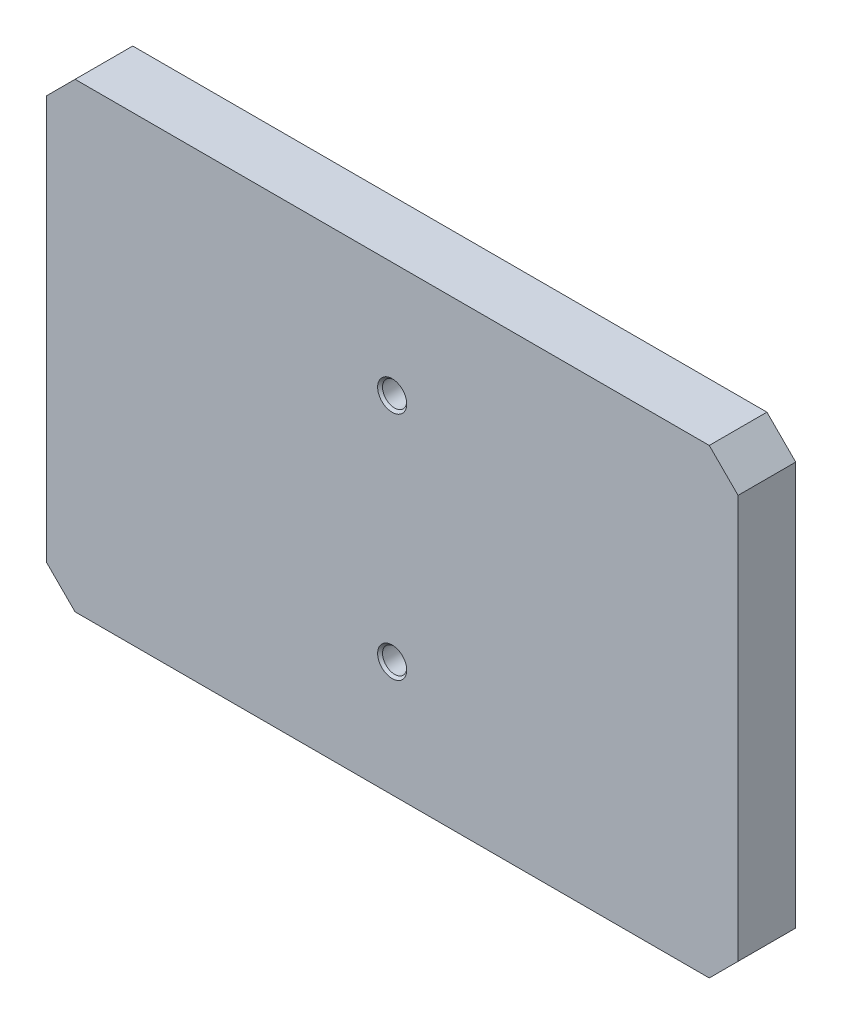
SolidWorks part; units mm, degrees
material "Q235-A "
ref_plane "前视基准面" through (0, 0, 0) normal (0, 0, 1) x (1, 0, 0)
ref_plane "上视基准面" through (0, 0, 0) normal (0, 1, 0) x (1, 0, 0)
ref_plane "右视基准面" through (0, 0, 0) normal (1, 0, 0) x (0, 0, -1)
sketch "草图1" plane through (0, 0, 0) normal (0, 0, 1) x (1, 0, 0)
  line L1 (-60, 40) -> (60, 40)
  line L2 (-60, 40) -> (-60, -40)
  line L3 (-60, -40) -> (60, -40)
  line L4 (60, 40) -> (60, -40)
  line L5 (-60, 40) -> (60, -40) construction
  line L6 (-60, -40) -> (60, 40) construction
  point P0 (0, 0)
  dimension "D1" = 80
  dimension "D2" = 120
extrude "凸台-拉伸1" add sketch "草图1" along normal blind 10
chamfer "倒角1" distance 5 angle 45 4 edges at (60, -40, 5) (-60, -40, 5) (60, 40, 5) (-60, 40, 5)
sketch "草图2" plane through (0, 0, 10) normal (0, 0, 1) x (1, 0, 0)
  line L0 (0, 40) -> (0, -40) construction
  line L1 (55, 40) -> (-55, 40) construction
  line L2 (-55, -40) -> (55, -40) construction
  line L3 (0, 0) -> (60, 0) construction
  line L4 (60, -35) -> (60, 35) construction
  circle A0 centre (0, 20) radius 2.5
  circle A1 centre (0, -20) radius 2.5
  dimension "D1" = 5
  dimension "D2" = 40
hole_wizard "M5 螺纹孔1" positions "3D草图1" profile "草图3" tap size "M5" standard "GB"
sketch3d "3D草图1"
  point P0 (0, 20, 10)
  point P3 (0, -20, 10)
sketch "草图3" plane through (0, 20, 10) normal (1, 0, 0) x (0, -1, 0)
  line L0 (0, 0) -> (0, 15.2618)
  line L1 (0, 15.2618) -> (2.1, 14)
  line L2 (2.1, 14) -> (2.1, 0.425)
  line L3 (2.1, 0.425) -> (2.525, 0)
  line L5 (2.525, 0) -> (0, 0)
  line L6 (-2.1, 0.425) -> (-2.525, 0) construction
  line L10 (0, 15.2618) -> (-2.1, 14) construction
  line L11 (0, -6.35) -> (0, 107.95) construction
  dimension "螺纹孔钻头直径" = 4.2
  dimension "螺纹孔钻头深度" = 14
  dimension "近端锥形沉头孔直径" = 5.05
  dimension "近端锥形沉头孔角度" = 90
  dimension "导头角度" = 118
cosmetic thread "孔螺蚊线1"
cosmetic thread "孔螺蚊线2"
